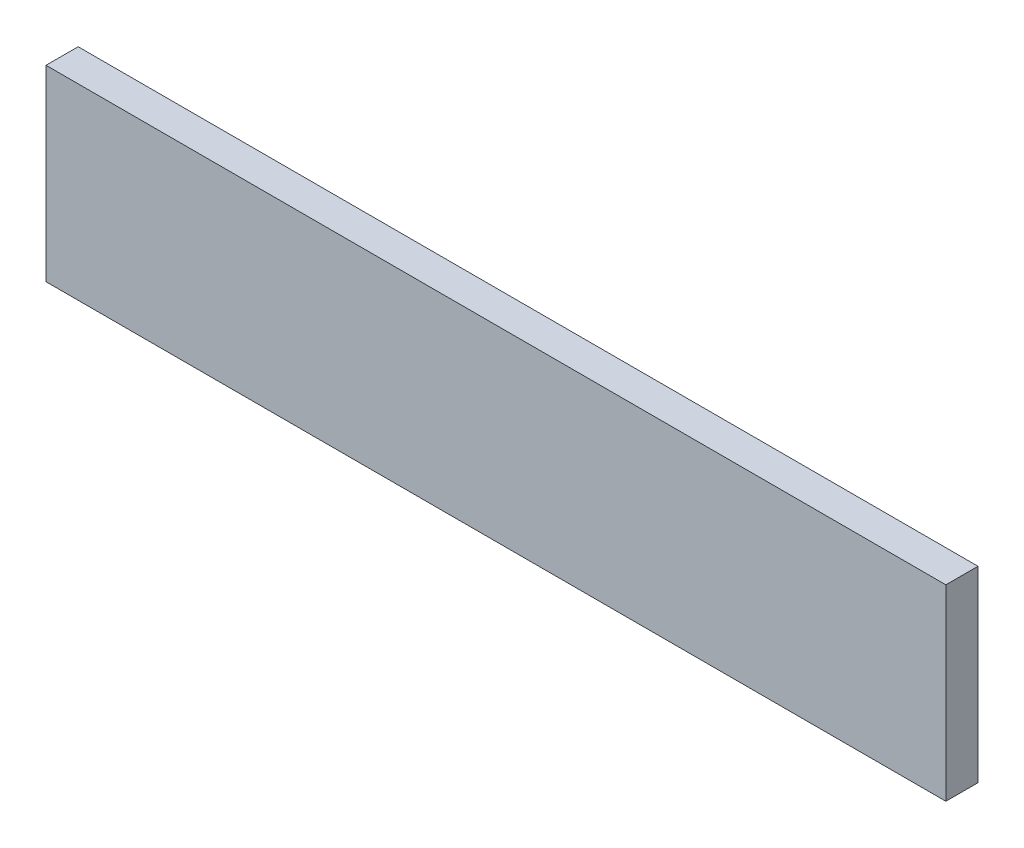
SolidWorks part; units mm, degrees
material "Q235B"
ref_plane "Front Plane" through (0, 0, 0) normal (0, 0, 1) x (1, 0, 0)
ref_plane "Top Plane" through (0, 0, 0) normal (0, 1, 0) x (1, 0, 0)
ref_plane "Right Plane" through (0, 0, 0) normal (1, 0, 0) x (0, 0, -1)
sketch "Sketch1" plane through (0, 0, 0) normal (0, 0, 1) x (1, 0, 0)
  line L1 (0, 0) -> (840, 0)
  line L2 (0, 0) -> (0, 175)
  line L3 (0, 175) -> (840, 175)
  line L4 (840, 0) -> (840, 175)
  dimension "D1" = 840
  dimension "D2" = 175
extrude "Boss-Extrude1" add sketch "Sketch1" along normal blind 30
